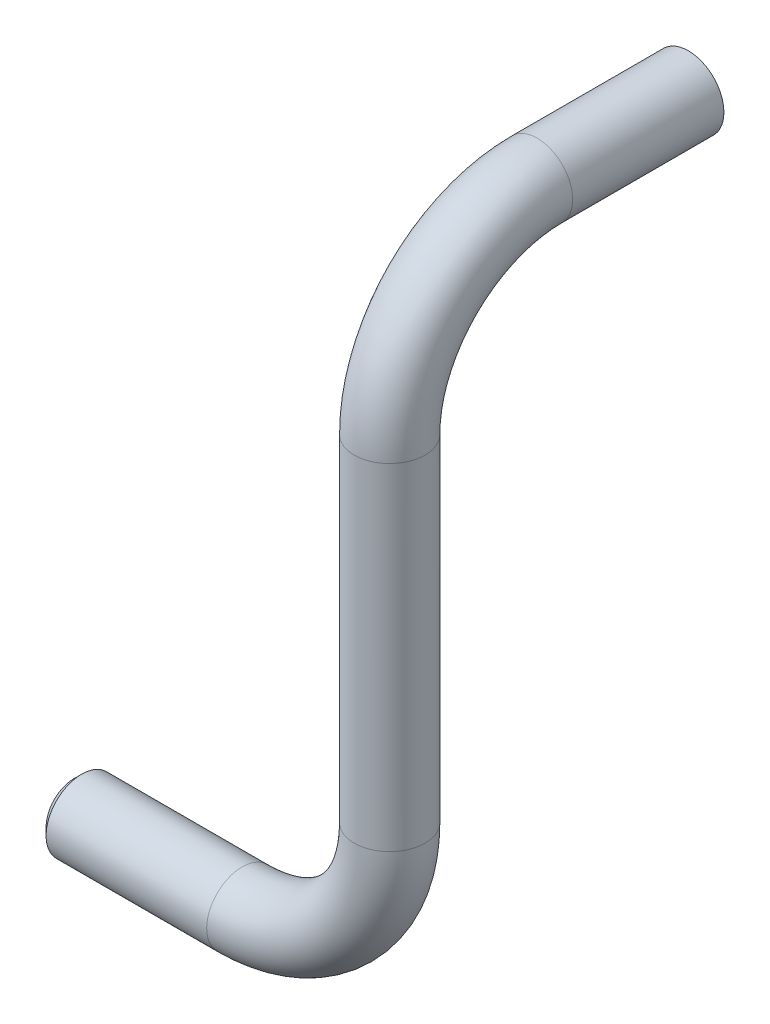
from build123d import *

# Parameters (mm, degrees)
SWEEP1_PROFILE_R = 9.5
CHAMFER1_SIZE    = 2


with BuildPart() as part:
    # Sweep1: sweep along a curve in space
    with BuildLine() as sweep1_path:
        Line((0, 0, 0), (0, 0, 40.5))
        ThreePointArc((0, 0, 40.5), (0, -11.569282143, 68.430717857), (0, -39.5, 80))
        Line((0, -39.5, 80), (0, -129.5, 80))
        ThreePointArc((0, -129.5, 80), (-11.569282143, -157.430717857, 80), (-39.5, -169, 80))
        Line((-39.5, -169, 80), (-84.5, -169, 80))
    # Sweep1 profile (on start of the path) → Sweep1 (sweep)
    with BuildSketch(Plane.XY):
        Circle(SWEEP1_PROFILE_R)
    sweep(path=sweep1_path.line)

    # Chamfer1
    chamfer1_edges = [part.edges().sort_by_distance(p)[0] for p in [
        (-84.5, -159.5, 80),
    ]]
    chamfer(chamfer1_edges, length=CHAMFER1_SIZE)


solid = part.part
